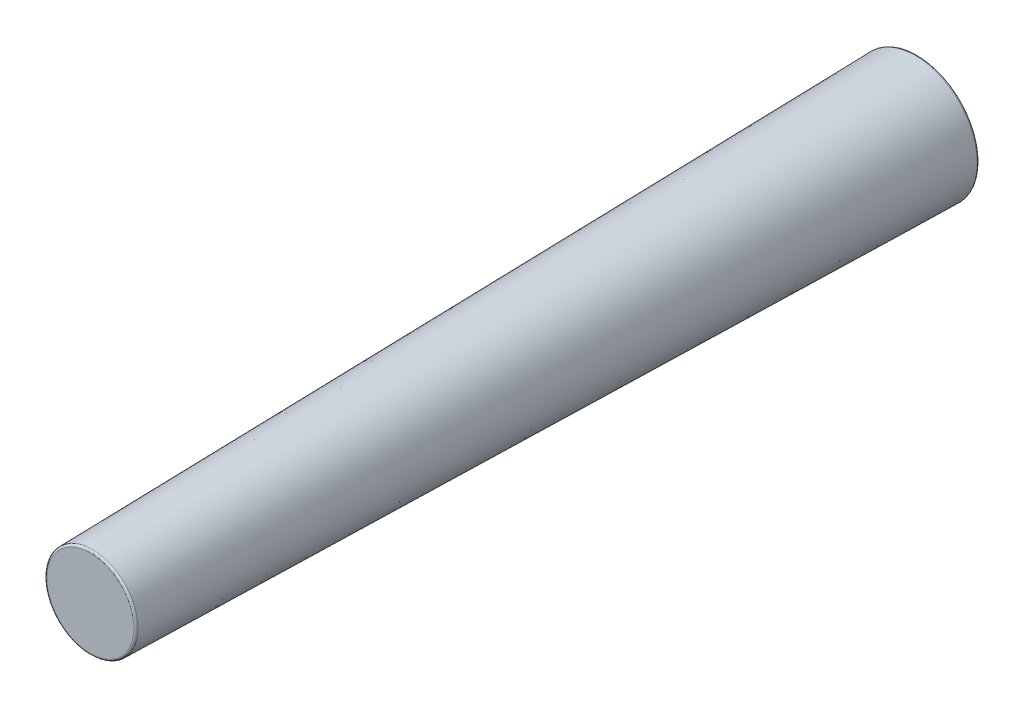
from build123d import *

# Parameters (mm, degrees)
SKETCH_1_R      = 3
EXTRUDE_1_DEPTH = 40
EXTRUDE_1_TAPER = 1.14
FILLET_1_R      = 0.1


with BuildPart() as part:
    # 草图1 → 凸台-拉伸1 (new body)
    with BuildSketch(Plane.XY):
        Circle(SKETCH_1_R)
    extrude(amount=EXTRUDE_1_DEPTH, taper=EXTRUDE_1_TAPER)

    # 圆角1
    fillet_1_edges = [part.edges().sort_by_distance(p)[0] for p in [
        (-3, 0, 0),
        (-2.204024821, 0, 40),
    ]]
    fillet(fillet_1_edges, radius=FILLET_1_R)


solid = part.part
